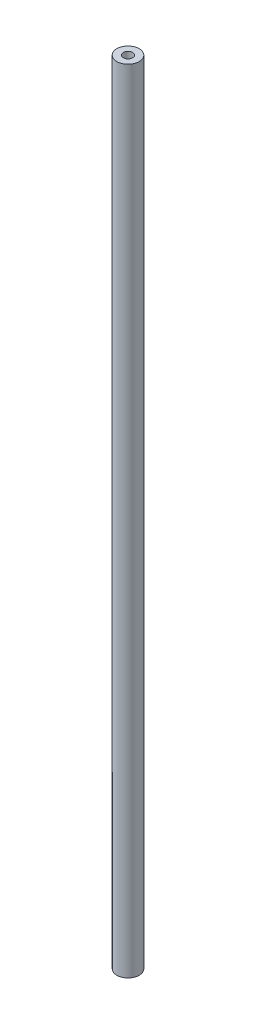
from build123d import *

# Parameters (mm, degrees)
SKETCH1_W = 0.7
SKETCH1_H = 85


with BuildPart() as part:
    # Sketch1 → Revolve1 (revolve)
    with BuildSketch(Plane.XY, mode=Mode.PRIVATE) as revolve1_sk:
        with Locations((-0.85, 42.5)):
            Rectangle(SKETCH1_W, SKETCH1_H)
    revolve(revolve1_sk.sketch.rotate(Axis((0, -6.441627678, 0), (0, 1, 0)), 270), axis=Axis((0, -6.441627678, 0), (0, 1, 0)))


solid = part.part
